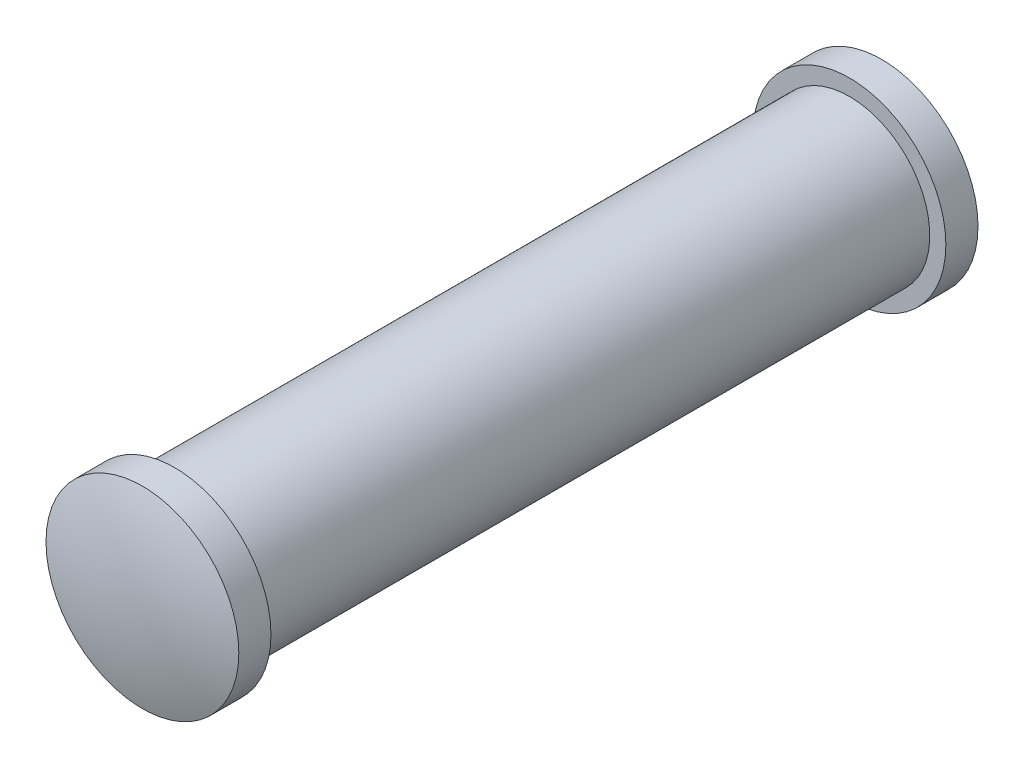
from build123d import *

# Parameters (mm, degrees)
SKETCH1_R           = 2.5
BOSS_EXTRUDE1_DEPTH = 10.5
SKETCH2_R           = 3
BOSS_EXTRUDE2_DEPTH = 1
BOSS_EXTRUDE3_START = 1
SKETCH3_R           = 3
BOSS_EXTRUDE3_DEPTH = 1
DOME1_FACE_RADIUS   = 3
DOME1_HEIGHT        = 0.5
DOME2_FACE_RADIUS   = 3
DOME2_HEIGHT        = 0.5


with BuildPart() as part:
    # Sketch1 → Boss-Extrude1 (new, symmetric)
    with BuildSketch(Plane.XY):
        with Locations(Location((0, 0, 0), (0, 0, 180))):
            Circle(SKETCH1_R)
    extrude(amount=BOSS_EXTRUDE1_DEPTH, both=True)

    # Sketch2 → Boss-Extrude2 (add)
    with BuildSketch(Plane(origin=(0, 0, -10.5), x_dir=(-1, 0, 0), z_dir=(0, 0, -1))):
        Circle(SKETCH2_R)
    extrude(amount=BOSS_EXTRUDE2_DEPTH)

    # Sketch3 → Boss-Extrude3 (add)
    with BuildSketch(Plane.XY.offset(10.5).offset(BOSS_EXTRUDE3_START)):
        with Locations(Location((0, 0, 0), (0, 0, 180))):
            Circle(SKETCH3_R)
    extrude(amount=-BOSS_EXTRUDE3_DEPTH)

    # Dome1: a dome of height H over a round flat face of radius A is a cap of a sphere of radius (A * A + H * H) / (2 * H)
    dome1_r = (DOME1_FACE_RADIUS * DOME1_FACE_RADIUS + DOME1_HEIGHT * DOME1_HEIGHT) / (2 * DOME1_HEIGHT)
    dome1_base = Plane((0, 0, -11.5), z_dir=(0, 0, -1))
    with Locations(dome1_base.offset(DOME1_HEIGHT - dome1_r)):
        dome1_ball = Sphere(dome1_r, mode=Mode.PRIVATE)
    add(split(dome1_ball, bisect_by=dome1_base, keep=Keep.TOP, mode=Mode.PRIVATE))

    # Dome2: a dome of height H over a round flat face of radius A is a cap of a sphere of radius (A * A + H * H) / (2 * H)
    dome2_r = (DOME2_FACE_RADIUS * DOME2_FACE_RADIUS + DOME2_HEIGHT * DOME2_HEIGHT) / (2 * DOME2_HEIGHT)
    dome2_base = Plane((0, 0, 11.5), z_dir=(0, 0, 1))
    with Locations(dome2_base.offset(DOME2_HEIGHT - dome2_r)):
        dome2_ball = Sphere(dome2_r, mode=Mode.PRIVATE)
    add(split(dome2_ball, bisect_by=dome2_base, keep=Keep.TOP, mode=Mode.PRIVATE))


solid = part.part
